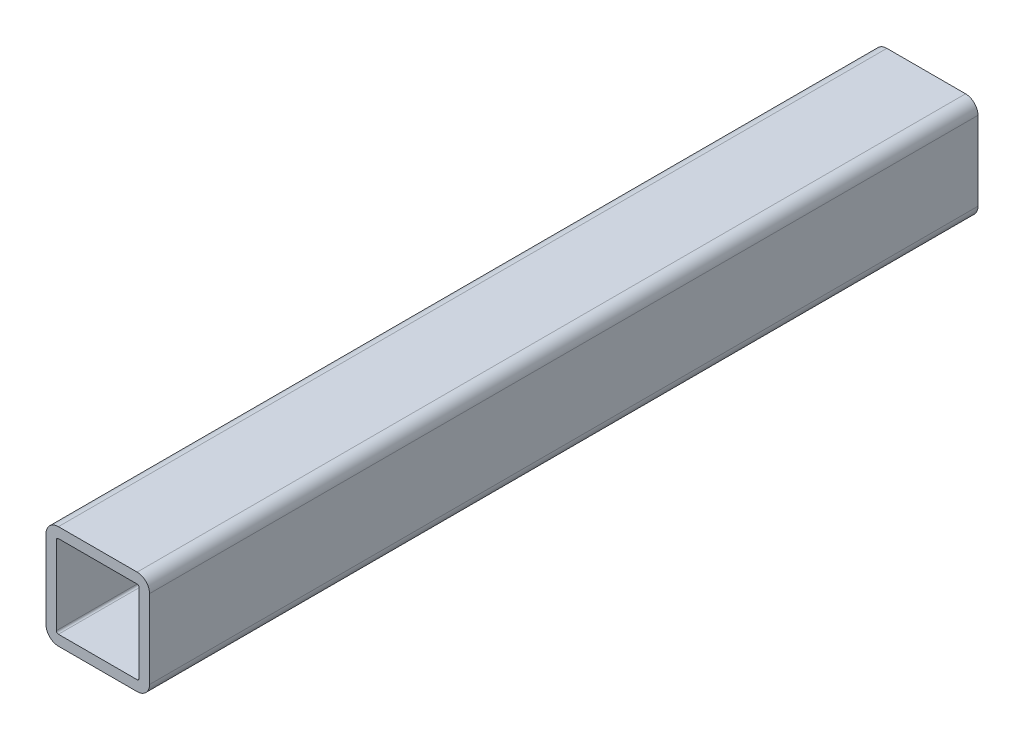
SolidWorks part; units mm, degrees
material "Q235B"
ref_plane "Front Plane" through (0, 0, 0) normal (0, 0, 1) x (1, 0, 0)
ref_plane "Top Plane" through (0, 0, 0) normal (0, 1, 0) x (1, 0, 0)
ref_plane "Right Plane" through (0, 0, 0) normal (1, 0, 0) x (0, 0, -1)
sketch "Sketch1" plane through (0, 0, 0) normal (0, 0, 1) x (1, 0, 0)
  line L0 (6, 45) -> (44, 45)
  line L1 (6, 0) -> (44, 0)
  line L2 (0, 6) -> (0, 44)
  line L3 (6, 50) -> (44, 50)
  line L4 (50, 6) -> (50, 44)
  line L5 (45, 6) -> (45, 44)
  line L6 (6, 5) -> (44, 5)
  line L7 (5, 6) -> (5, 44)
  arc A0 (6, 0) -> (0, 6) centre (6, 6) cw
  arc A1 (44, 0) -> (50, 6) centre (44, 6) ccw
  arc A2 (44, 50) -> (50, 44) centre (44, 44) cw
  arc A3 (0, 44) -> (6, 50) centre (6, 44) cw
  arc A4 (5, 44) -> (6, 45) centre (6, 44) cw
  arc A5 (44, 45) -> (45, 44) centre (44, 44) cw
  arc A6 (44, 5) -> (45, 6) centre (44, 6) ccw
  arc A7 (6, 5) -> (5, 6) centre (6, 6) cw
  point P7 (0, 0)
  point P12 (50, 50)
  point P15 (0, 50)
  dimension "D3" = 6
  dimension "D1" = 50
  dimension "D2" = 50
  dimension "D4" = 5
extrude "Boss-Extrude1" add sketch "Sketch1" along normal blind 400
